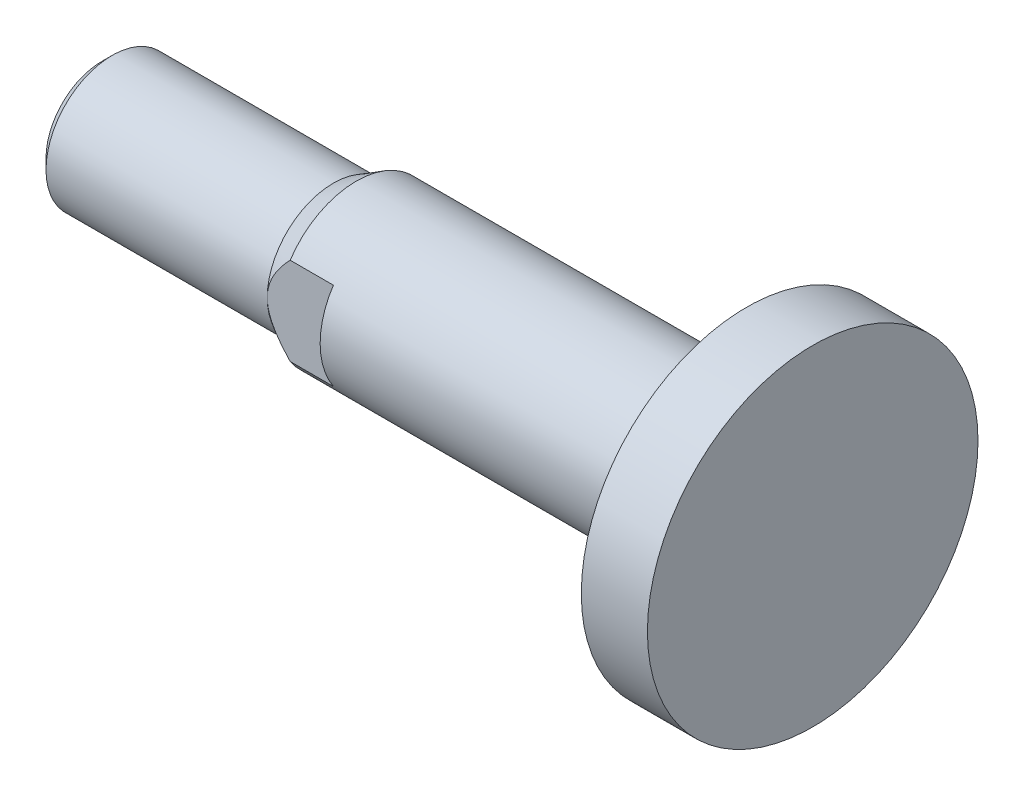
from build123d import *

# Parameters (mm, degrees)
SKETCH2_R          = 12
SKETCH2_W          = 10
SKETCH2_H          = 14
CUT_EXTRUDE1_DEPTH = 5


with BuildPart() as part:
    # Sketch1 → Revolve1 (revolve)
    with BuildSketch(Plane.XY, mode=Mode.PRIVATE) as revolve1_sk:
        Polygon((-22.5, 0), (-22.5, 4.233), (-21.733, 5), (-5, 5), (-3.267949192, 6), (26.25, 6), (26.25, 12.5), (31.25, 12.5), (31.25, 0), align=None)
    revolve(revolve1_sk.sketch.rotate(Axis((31.25, 0, 0), (-1, 0, 0)), 270), axis=Axis((31.25, 0, 0), (-1, 0, 0)))

    # Sketch2 → Cut-Extrude1 (cut)
    with BuildSketch(Plane(origin=(0, 0, 0), x_dir=(0, 0, -1), z_dir=(1, 0, 0))):
        Circle(SKETCH2_R)
        Rectangle(SKETCH2_W, SKETCH2_H, mode=Mode.SUBTRACT)
    extrude(amount=-CUT_EXTRUDE1_DEPTH, mode=Mode.SUBTRACT)


solid = part.part
